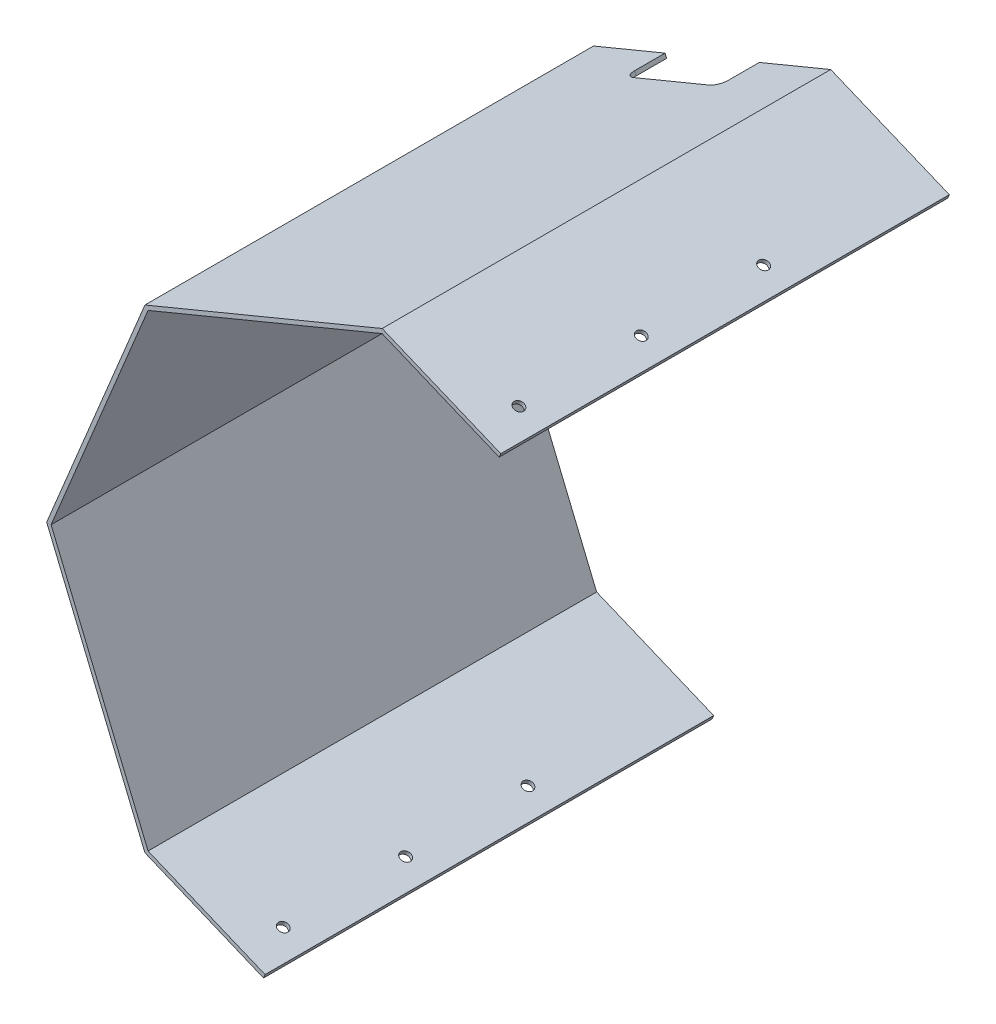
from build123d import *

# Parameters (mm, degrees)
BOSS_EXTRUDE1_DEPTH = 220
SHELL1_T            = -2
CUT_EXTRUDE1_DEPTH  = 321.212491043
SKETCH3_R           = 2.5
CUT_EXTRUDE2_DEPTH  = 394.612153142
SKETCH4_W           = 20
SKETCH4_H           = 30
CUT_EXTRUDE3_DEPTH  = 357.766015962
FILLET1_R           = 5
SKETCH5_W           = 50
SKETCH5_H           = 20
CUT_EXTRUDE4_DEPTH  = 376.254580252
FILLET2_R           = 5


with BuildPart() as part:
    # Sketch1 → Boss-Extrude1 (new body)
    with BuildSketch(Plane.XY):
        Polygon((-164.523614444, 0), (-116.335763439, -116.335763439), (0, -164.523614444), (116.335763439, -116.335763439), (164.523614444, 0), (116.335763439, 116.335763439), (0, 164.523614444), (-116.335763439, 116.335763439), align=None)
    extrude(amount=BOSS_EXTRUDE1_DEPTH)

    # Shell1
    shell1_openings = [part.faces().sort_by_distance(p)[0] for p in [
        (0, 0, 220),
        (0, 0, 0),
    ]]
    offset(amount=SHELL1_T, openings=shell1_openings, kind=Kind.INTERSECTION)

    # Sketch2 → Cut-Extrude1 (cut, through all)
    with BuildSketch(Plane.XY.offset(220)):
        Polygon((75.61693775, 182.555436661), (-82.042454152, -198.068005503), (95.714298716, -271.697263345), (253.373690618, 108.92617882), align=None)
    extrude(amount=-CUT_EXTRUDE1_DEPTH, mode=Mode.SUBTRACT)

    # Sketch3 → Cut-Extrude2 (cut, through all)
    with BuildSketch(Plane(origin=(-58.167881719, -140.429688942, 0), x_dir=(0.9238795325112961, -0.3826834323650676, 0), z_dir=(-0.3826834323650675, -0.923879532511296, 0))):
        with Locations((-12, 200)):
            Circle(SKETCH3_R)
        with Locations((-12, 140)):
            Circle(SKETCH3_R)
        with Locations((-12, 80)):
            Circle(SKETCH3_R)
    extrude(amount=-CUT_EXTRUDE2_DEPTH, mode=Mode.SUBTRACT)

    # Sketch4 → Cut-Extrude3 (cut, through all)
    with BuildSketch(Plane(origin=(-140.429688942, 58.167881719, 0), x_dir=(0, 0, 1), z_dir=(-0.9238795325112957, 0.3826834323650681, 0))):
        with Locations((10, -37.960461481)):
            Rectangle(SKETCH4_W, SKETCH4_H)
    extrude(amount=-CUT_EXTRUDE3_DEPTH, mode=Mode.SUBTRACT)

    # Fillet1
    fillet1_edges = [part.edges().sort_by_distance(p)[0] for p in [
        (-148.292397617, 36.572497868, 20),
        (-159.772900588, 8.856111893, 20),
    ]]
    fillet(fillet1_edges, radius=FILLET1_R)

    # Sketch5 → Cut-Extrude4 (cut, through all)
    with BuildSketch(Plane(origin=(-58.167881719, 140.429688942, 0), x_dir=(0.9238795325112777, 0.3826834323651116, 0), z_dir=(-0.38268343236511165, 0.9238795325112779, 0))):
        with Locations((0.039538519, -10)):
            Rectangle(SKETCH5_W, SKETCH5_H)
    extrude(amount=-CUT_EXTRUDE4_DEPTH, mode=Mode.SUBTRACT)

    # Fillet2
    fillet2_edges = [part.edges().sort_by_distance(p)[0] for p in [
        (-34.651681146, 149.088025955, 20),
        (-80.845657771, 129.953854336, 20),
    ]]
    fillet(fillet2_edges, radius=FILLET2_R)


solid = part.part
